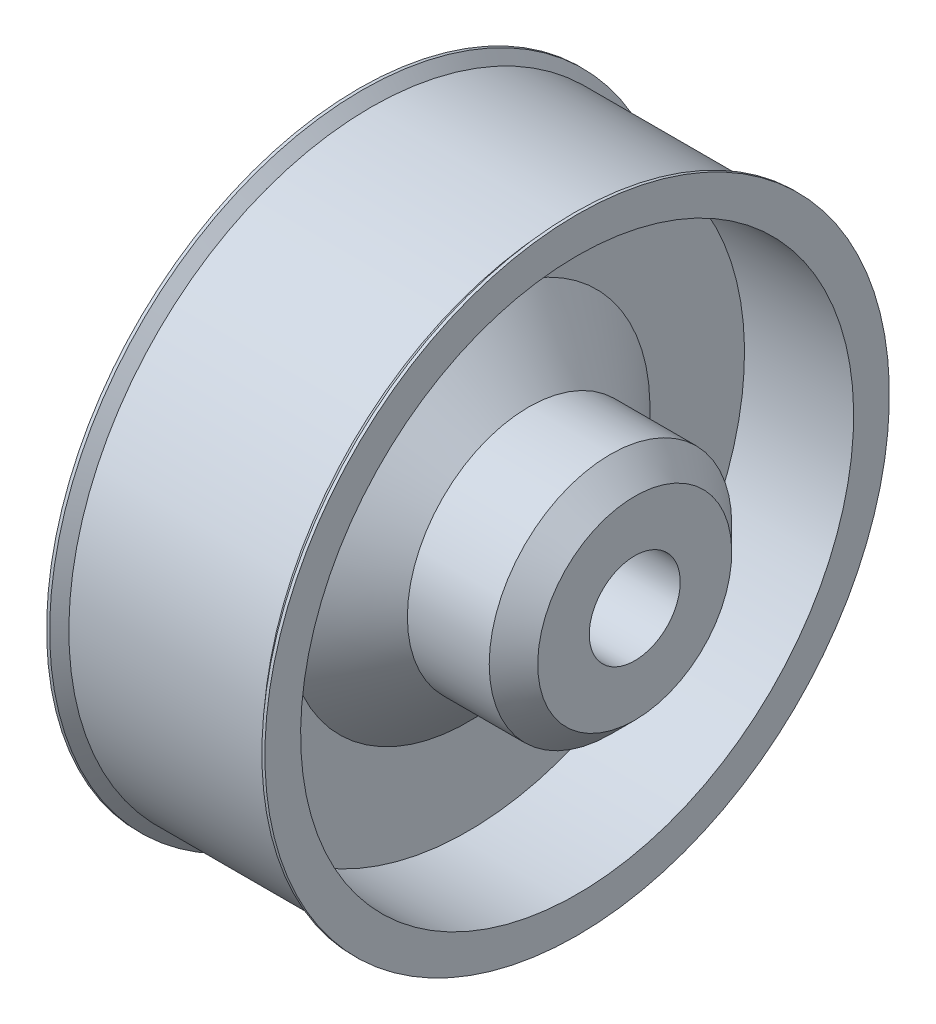
SolidWorks part; units mm, degrees
ref_plane "Front Plane" through (0, 0, 0) normal (0, 0, 1) x (1, 0, 0)
ref_plane "Top Plane" through (0, 0, 0) normal (0, 1, 0) x (1, 0, 0)
ref_plane "Right Plane" through (0, 0, 0) normal (1, 0, 0) x (0, 0, -1)
other "Configuration Table"
sketch "Sketch1" plane through (0, 0, 0) normal (0, 0, 1) x (1, 0, 0)
  line L0 (0, 0) -> (0, 0.375)
  line L1 (0, 0.375) -> (1.05, 0.6)
  line L2 (1.05, 0.6) -> (1.05, 1.2938)
  line L3 (1.05, 3.3062) -> (1.05, 4.2312)
  line L8 (0.7206, 4.5606) -> (0, 4.5606)
  line L9 (0, 4.5606) -> (0, 5.15)
  line L11 (0.2, 4.9829) -> (3.4, 4.9829)
  line L13 (3.6, 5.15) -> (3.6, 4.5606)
  line L14 (3.6, 4.5606) -> (1.8, 4.5606)
  line L15 (1.8, 4.5606) -> (1.8, 2)
  line L17 (1.8, 2) -> (4.55, 2)
  line L19 (4.55, 2) -> (4.55, 0.75)
  line L20 (4.55, 0.75) -> (1.8, 0.75)
  line L21 (1.8, 0.75) -> (1.8, 0)
  line L22 (1.8, 0) -> (0, 0)
  line L23 (0.2, 4.9829) -> (0.05, 5.15)
  line L24 (3.4, 4.9829) -> (3.55, 5.15)
  line L25 (3.55, 5.15) -> (3.6, 5.15)
  line L26 (0.05, 5.15) -> (0, 5.15)
  arc A0 (1.05, 1.2938) -> (0.8357, 1.5813) centre (0.75, 1.2938) ccw
  arc A1 (0.8357, 1.5813) -> (0.8357, 3.0187) centre (1.05, 2.3) cw
  arc A2 (0.8357, 3.0187) -> (1.05, 3.3062) centre (0.75, 3.3062) ccw
  arc A4 (1.05, 4.2312) -> (0.7206, 4.5606) centre (0.7206, 4.2312) ccw
  dimension "D1" = 0.75
  dimension "D10" = 0.3
  dimension "D11" = 0.3
  dimension "D12" = 0.3294
  dimension "D15" = 0.75
  dimension "D2" = 2
  dimension "D3" = 3.2
  dimension "D4" = 1.05
  dimension "D5" = 2.3
  dimension "D6" = 0.4223
  dimension "D7" = 0.1671
  dimension "D8" = 4.55
  dimension "D9" = 1.8
  dimension "D13" = 5.15
  dimension "D14" = 0.75
  dimension "D16" = 3.6
  dimension "D17" = 1.8
  dimension "D18" = 0.15
  dimension "D19" = 0.375
  dimension "D20" = 0.6
  dimension "D21" = 0.15
  dimension "D22" = 0.05
revolve "Revolve1" add sketch "Sketch1" angle 360 about L22
chamfer "Chamfer1" distance 0.4 angle 45 1 edges at (4.55, 2, 0)
fillet "Fillet1" radius 0.2 1 edges at (0, 4.5606, 0)
chamfer "Chamfer2" distance 1 angle 45 1 edges at (1.8, 2, 0)
sketch "Sketch2" plane through (1.05, 0, 0) normal (-1, 0, 0) x (0, 0, 1)
  line L1 (0.2887, 3.76) -> (0.1443, 4.01)
  line L2 (0.1443, 4.01) -> (-0.1443, 4.01)
  line L3 (-0.1443, 4.01) -> (-0.2887, 3.76)
  line L4 (-0.2887, 3.76) -> (-0.1443, 3.51)
  line L5 (-0.1443, 3.51) -> (0.1443, 3.51)
  line L6 (0.1443, 3.51) -> (0.2887, 3.76)
  circle A0 centre (0, 3.76) radius 0.25 construction
  dimension "D1" = 3.76
  dimension "D2" = 0.5
extrude "Boss-Extrude1" add sketch "Sketch2" along normal mid plane 0.3
pattern_circular "CirPattern1" count 8 over 360 about axis through (0, 0, 0) along (1, 0, 0) of "Boss-Extrude1"
sketch "Sketch3" plane through (1.05, 0, 0) normal (-1, 0, 0) x (0, 0, 1)
  line L1 (0.2887, 1) -> (0.1443, 1.25)
  line L2 (0.1443, 1.25) -> (-0.1443, 1.25)
  line L3 (-0.1443, 1.25) -> (-0.2887, 1)
  line L4 (-0.2887, 1) -> (-0.1443, 0.75)
  line L5 (-0.1443, 0.75) -> (0.1443, 0.75)
  line L6 (0.1443, 0.75) -> (0.2887, 1)
  circle A0 centre (0, 1) radius 0.25 construction
  dimension "D1" = 1
  dimension "D2" = 0.5
extrude "Boss-Extrude2" add sketch "Sketch3" along normal mid plane 0.3
pattern_circular "CirPattern2" count 5 over 360 about axis through (0, 0, 0) along (1, 0, 0) of "Boss-Extrude2"
